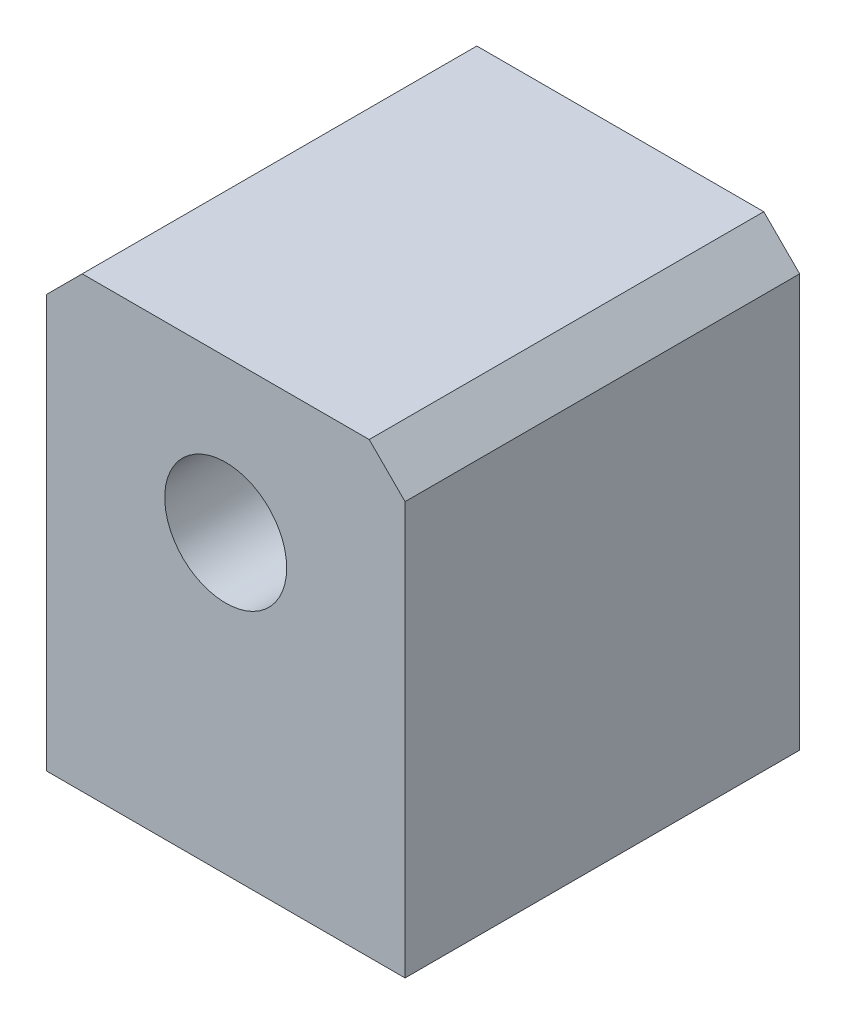
from build123d import *

# Parameters (mm, degrees)
SKETCH1_W                    = 20
SKETCH1_H                    = 25
BOSS_EXTRUDE1_DEPTH          = 11
CHAMFER1_SIZE                = 2
M8_TAPPED_HOLE1_D            = 6.8
M4_TAPPED_HOLE1_D            = 3.3
M4_TAPPED_HOLE1_DEPTH        = 11.5
M4_TAPPED_HOLE1_TIP          = 0.991420021
F_4_0_4_DIAMETER_HOLE1_D     = 4
F_4_0_4_DIAMETER_HOLE1_DEPTH = 8
F_4_0_4_DIAMETER_HOLE1_TIP   = 1.201721238


with BuildPart() as part:
    # Sketch1 → Boss-Extrude1 (new, symmetric)
    with BuildSketch(Plane.XY):
        Rectangle(SKETCH1_W, SKETCH1_H)
    extrude(amount=BOSS_EXTRUDE1_DEPTH, both=True)

    # Chamfer1
    chamfer1_edges = [part.edges().sort_by_distance(p)[0] for p in [
        (-10, 12.5, 0),
        (10, 12.5, 0),
    ]]
    chamfer(chamfer1_edges, length=CHAMFER1_SIZE)

    # M8 Tapped Hole1 (through all)
    with Locations(Plane.XY.offset(11)):
        with Locations((0, 4)):
            Hole(M8_TAPPED_HOLE1_D / 2)

    # M4 Tapped Hole1
    with Locations(Plane(origin=(0, -12.5, 0), x_dir=(-1, 0, 0), z_dir=(0, -1, 0))):
        with Locations((6, -7), (-6, 7)):
            Hole(M4_TAPPED_HOLE1_D / 2, depth=M4_TAPPED_HOLE1_DEPTH)
            with Locations((0, 0, -(M4_TAPPED_HOLE1_DEPTH + M4_TAPPED_HOLE1_TIP / 2))):  # 118° drill point
                Cone(0, M4_TAPPED_HOLE1_D / 2, M4_TAPPED_HOLE1_TIP, mode=Mode.SUBTRACT)

    # Ø4.0 (4) Diameter Hole1
    with Locations(Plane(origin=(0, -12.5, 0), x_dir=(-1, 0, 0), z_dir=(0, -1, 0))):
        with Locations((-6, -7), (6, 7)):
            Hole(F_4_0_4_DIAMETER_HOLE1_D / 2, depth=F_4_0_4_DIAMETER_HOLE1_DEPTH)
            with Locations((0, 0, -(F_4_0_4_DIAMETER_HOLE1_DEPTH + F_4_0_4_DIAMETER_HOLE1_TIP / 2))):  # 118° drill point
                Cone(0, F_4_0_4_DIAMETER_HOLE1_D / 2, F_4_0_4_DIAMETER_HOLE1_TIP, mode=Mode.SUBTRACT)


solid = part.part
